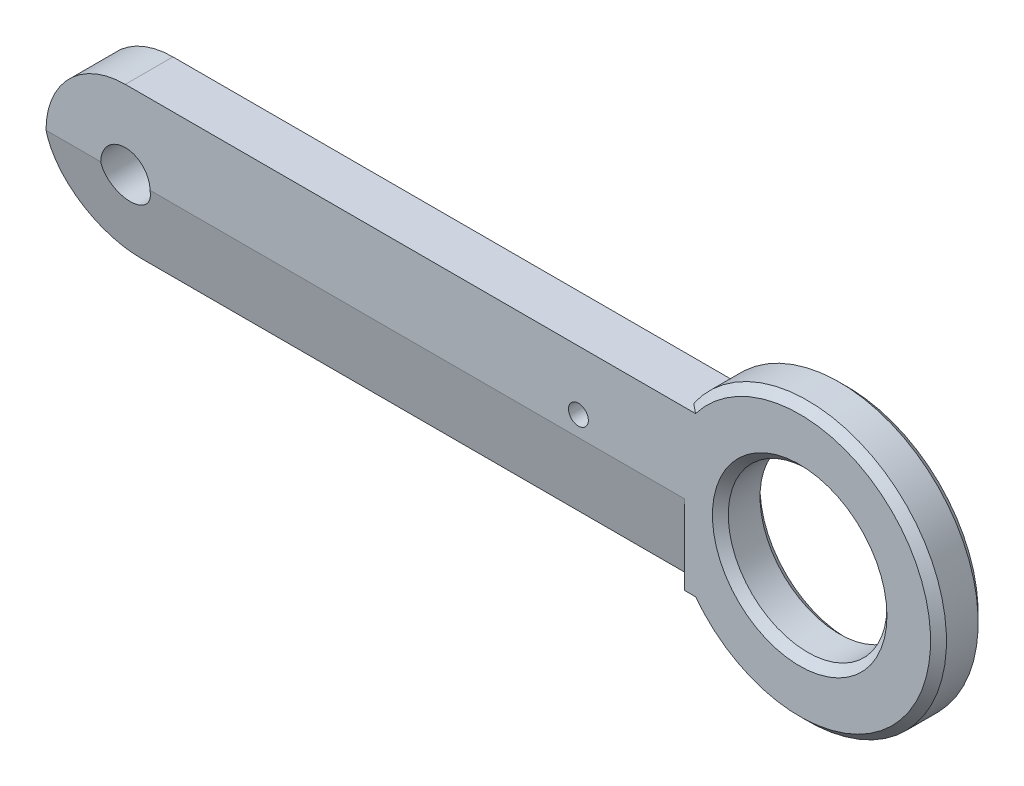
from build123d import *

# Parameters (mm, degrees)
SKETCH_6_R             = 17.5
EXTRUDE_3_DEPTH        = 6
SKETCH_7_R             = 10
CUT_EXTRUDE_1_DEPTH    = 10
SKETCH_8_R             = 3.1
CUT_EXTRUDE_2_DEPTH    = 10
CUT_EXTRUDE_3_DEPTH    = 83.598426135
CHAMFER_1_SIZE         = 1
HOLE_WIZARD_M3_1_D     = 2.5
HOLE_WIZARD_M3_1_DEPTH = 8.5
HOLE_WIZARD_M3_1_TIP   = 0.751075774


with BuildPart() as part:
    # 草图6 → 凸台-拉伸3 (new body)
    with BuildSketch(Plane.XY):
        with Locations((42.5, 0)):
            Circle(SKETCH_6_R)
        with BuildLine():
            Line((-42.5, 10), (42.5, 10))
            ThreePointArc((42.5, 10), (52.5, 0), (42.5, -10))
            Line((42.5, -10), (-42.5, -10))
            ThreePointArc((-42.5, -10), (-52.5, 0), (-42.5, 10))
        make_face()
    extrude(amount=EXTRUDE_3_DEPTH)

    # 草图7 → 切除-拉伸1 (cut)
    with BuildSketch(Plane(origin=(0, 0, 0), x_dir=(-1, 0, 0), z_dir=(0, 0, -1))):
        with Locations((-42.5, 0)):
            Circle(SKETCH_7_R)
    extrude(amount=-CUT_EXTRUDE_1_DEPTH, mode=Mode.SUBTRACT)

    # 草图8 → 切除-拉伸2 (cut)
    with BuildSketch(Plane(origin=(0, 0, 0), x_dir=(-1, 0, 0), z_dir=(0, 0, -1))):
        with Locations((42.5, 0)):
            Circle(SKETCH_8_R)
    extrude(amount=-CUT_EXTRUDE_2_DEPTH, mode=Mode.SUBTRACT)

    # 草图9 → 切除-拉伸3 (cut, through all)
    with BuildSketch(Plane(origin=(28, 0, 0), x_dir=(0, 0, -1), z_dir=(1, 0, 0))):
        Polygon((-4, -10), (-6, 0), (-6, -10), align=None)
        Polygon((-2, -10), (0, 0), (0, -10), align=None)
    extrude(amount=-CUT_EXTRUDE_3_DEPTH, mode=Mode.SUBTRACT)

    # 倒角1
    chamfer_1_edges = [part.edges().sort_by_distance(p)[0] for p in [
        (60, 0, 6),
        (52.5, 0, 6),
        (52.5, 0, 0),
        (60, 0, 0),
    ]]
    chamfer(chamfer_1_edges, length=CHAMFER_1_SIZE)

    # M3 螺纹孔1
    with Locations(Plane(origin=(0, 0, 0), x_dir=(-1, 0, 0), z_dir=(0, 0, -1))):
        with Locations((-14.611830465, 2.5)):
            Hole(HOLE_WIZARD_M3_1_D / 2, depth=HOLE_WIZARD_M3_1_DEPTH)
            with Locations((0, 0, -(HOLE_WIZARD_M3_1_DEPTH + HOLE_WIZARD_M3_1_TIP / 2))):  # 118° drill point
                Cone(0, HOLE_WIZARD_M3_1_D / 2, HOLE_WIZARD_M3_1_TIP, mode=Mode.SUBTRACT)


solid = part.part
